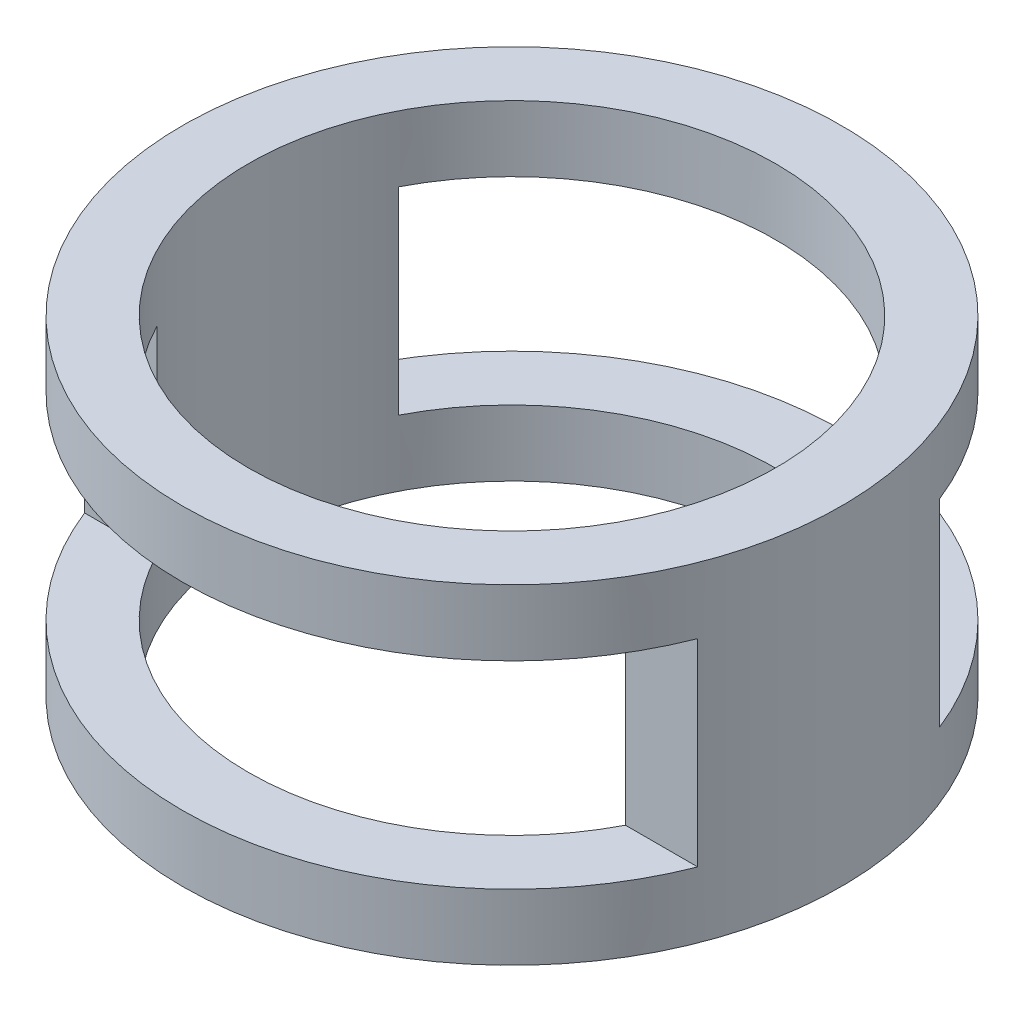
SolidWorks part; units mm, degrees
ref_plane "Front Plane" through (0, 0, 0) normal (0, 0, 1) x (1, 0, 0)
ref_plane "Top Plane" through (0, 0, 0) normal (0, 1, 0) x (1, 0, 0)
ref_plane "Right Plane" through (0, 0, 0) normal (1, 0, 0) x (0, 0, -1)
other "Configuration Table"
sketch "Sketch1" plane through (0, 0, 0) normal (0, 1, 0) x (1, 0, 0)
  circle A0 centre (0, 0) radius 30
  circle A1 centre (0, 0) radius 24
  dimension "D1" = 60
  dimension "D2" = 48
extrude "Boss-Extrude1" add sketch "Sketch1" along normal blind 30
sketch "Sketch2" plane through (0, 0, 0) normal (1, 0, 0) x (0, 0, -1)
  line L0 (-31.6089, 15) -> (35.3301, 15) construction
  line L1 (30, 30) -> (30, 0) construction
  line L2 (-30, 30) -> (-30, 0) construction
  line L3 (-49, 6) -> (-11, 6)
  line L4 (-49, 6) -> (-49, 24)
  line L5 (-49, 24) -> (-11, 24)
  line L6 (-11, 6) -> (-11, 24)
  line L7 (-49, 6) -> (-11, 24) construction
  line L8 (-49, 24) -> (-11, 6) construction
  line L9 (0, 0) -> (0, 35.4258) construction
  line L10 (-30, 0) -> (30, 0) construction
  line L11 (49, 6) -> (49, 24)
  line L12 (49, 6) -> (11, 6)
  line L13 (11, 6) -> (11, 24)
  line L14 (49, 24) -> (11, 24)
  point P6 (30, 15)
  point P7 (-30, 15)
  dimension "D1" = 18
  dimension "D2" = 11
extrude "Cut-Extrude1" cut sketch "Sketch2" against normal through all and the other way through all
